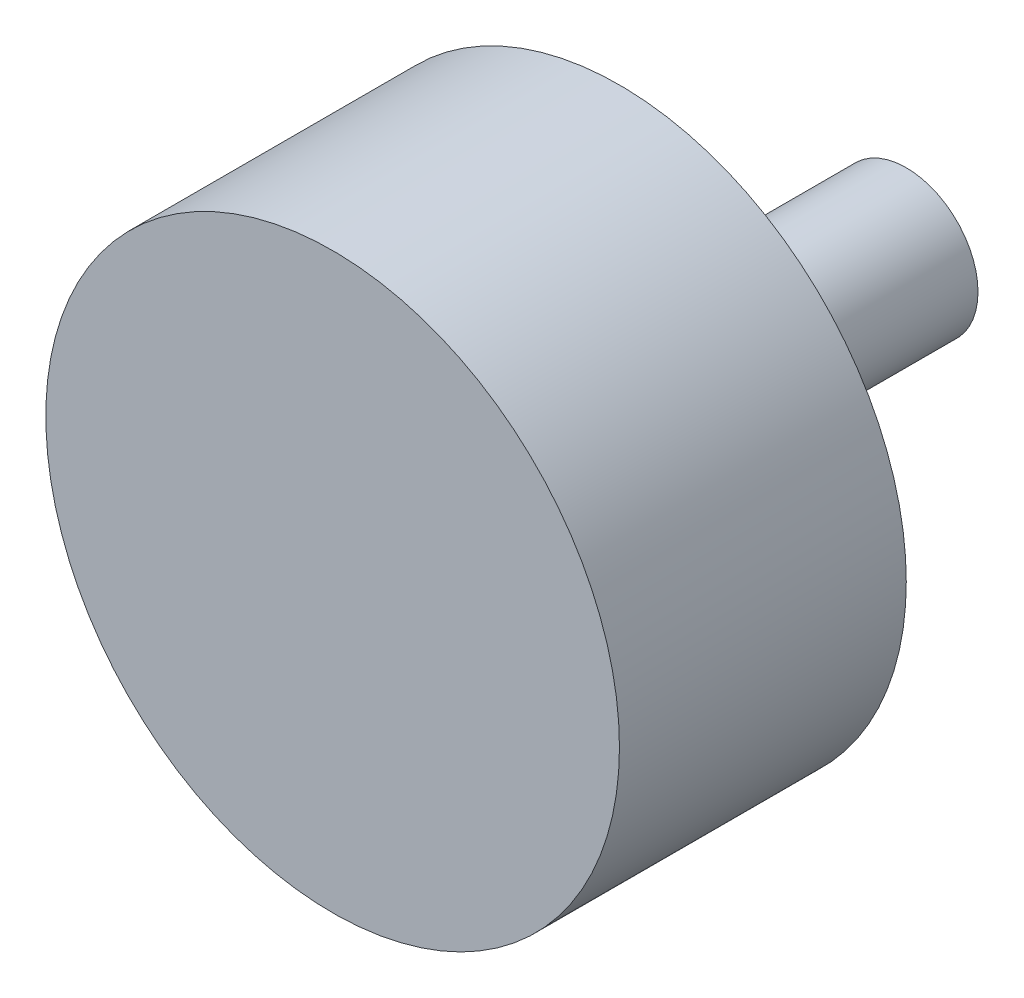
from build123d import *

# Parameters (mm, degrees)
SKETCH1_R           = 2.5
BOSS_EXTRUDE1_DEPTH = 10
SKETCH2_R           = 10
BOSS_EXTRUDE2_DEPTH = 10


with BuildPart() as part:
    # Sketch1 → Boss-Extrude1 (new body)
    with BuildSketch(Plane.XY):
        Circle(SKETCH1_R)
    extrude(amount=BOSS_EXTRUDE1_DEPTH)

    # Sketch2 → Boss-Extrude2 (add)
    with BuildSketch(Plane.XY.offset(10)):
        Circle(SKETCH2_R)
    extrude(amount=BOSS_EXTRUDE2_DEPTH)


solid = part.part
